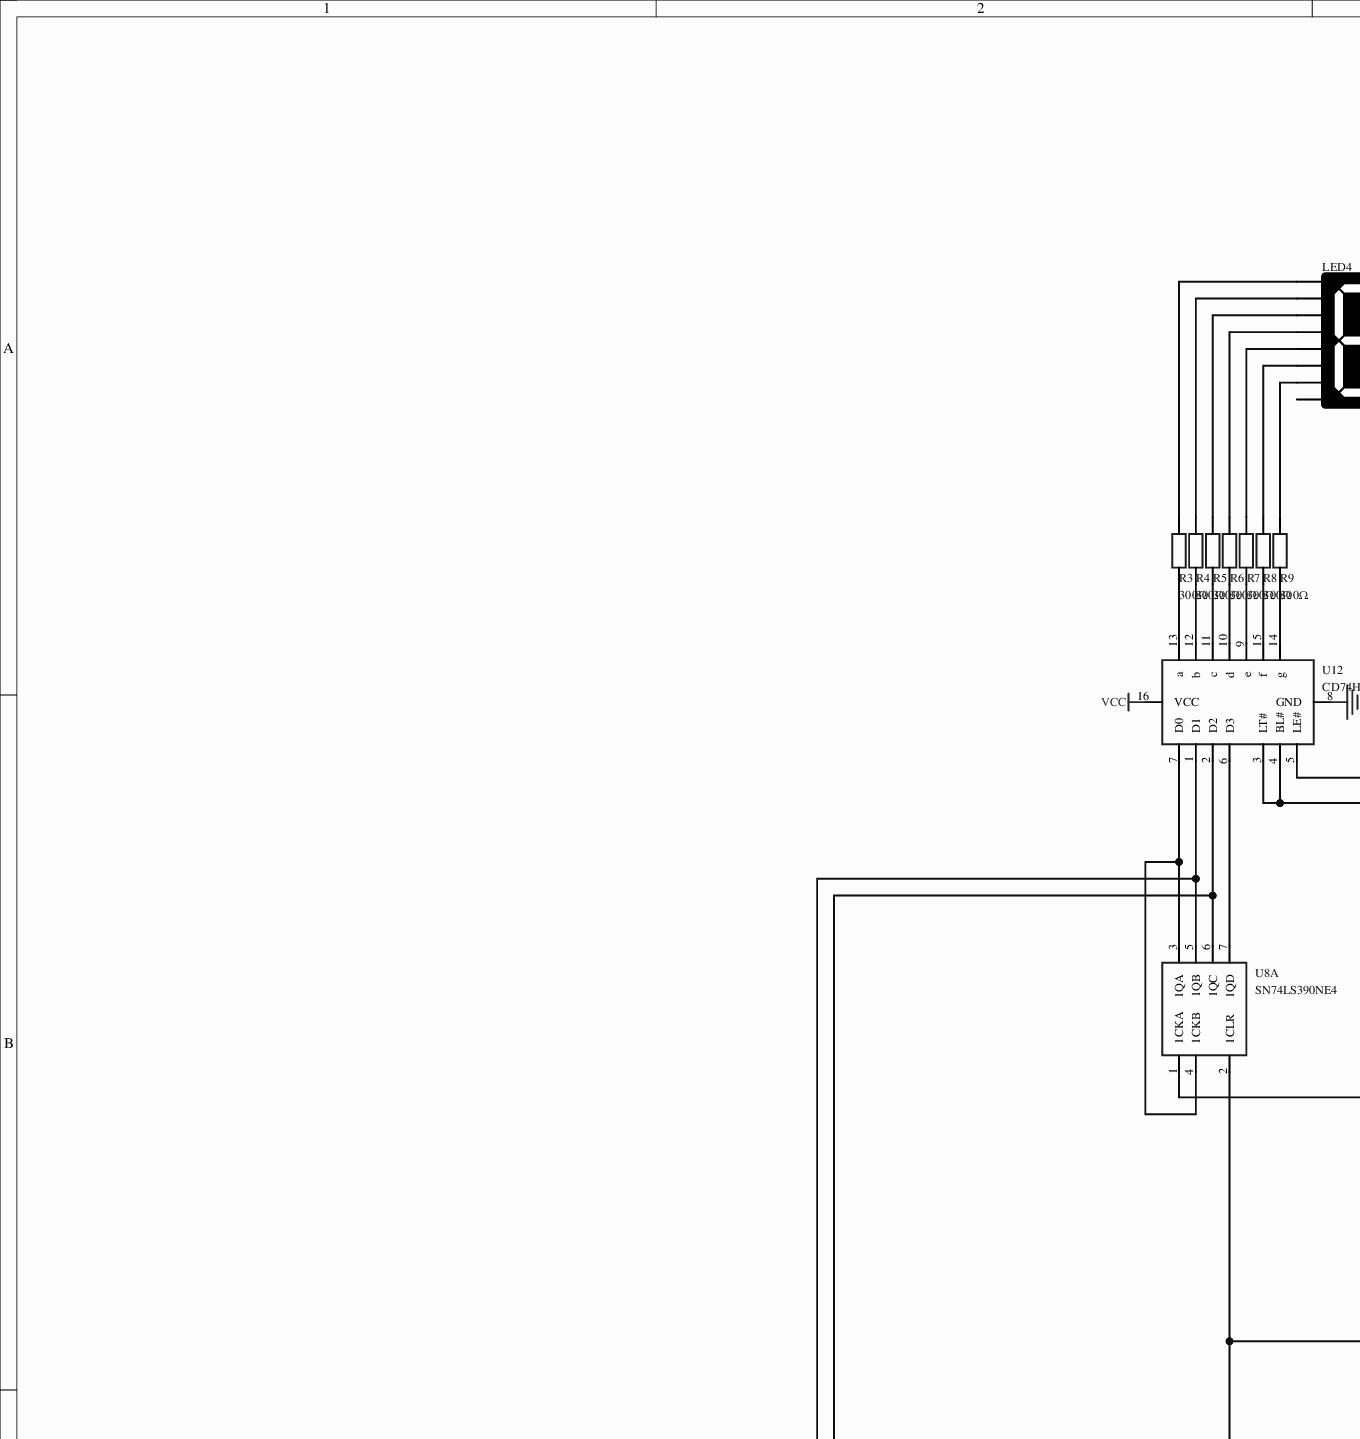
[diagram p0: MISC75414-3.schdoc, top left]
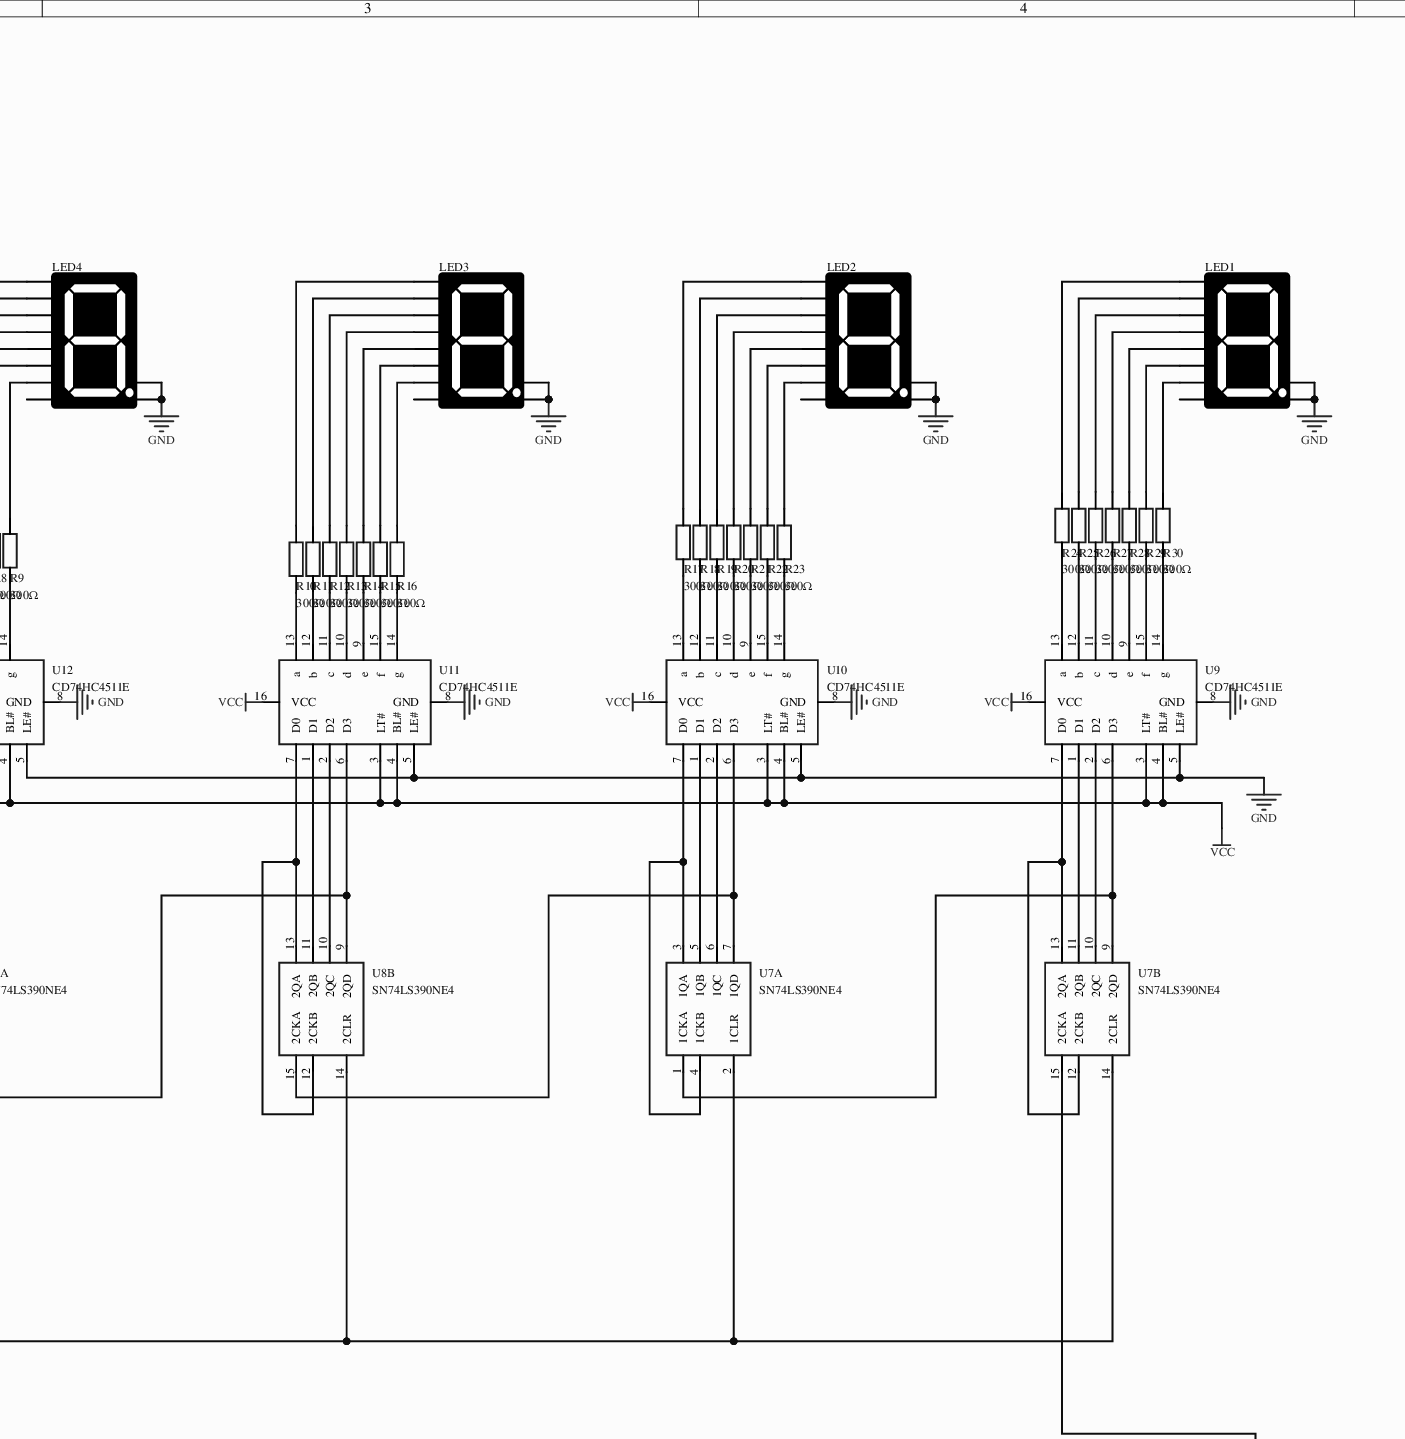
[diagram p1: MISC75414-3.schdoc, top middle]
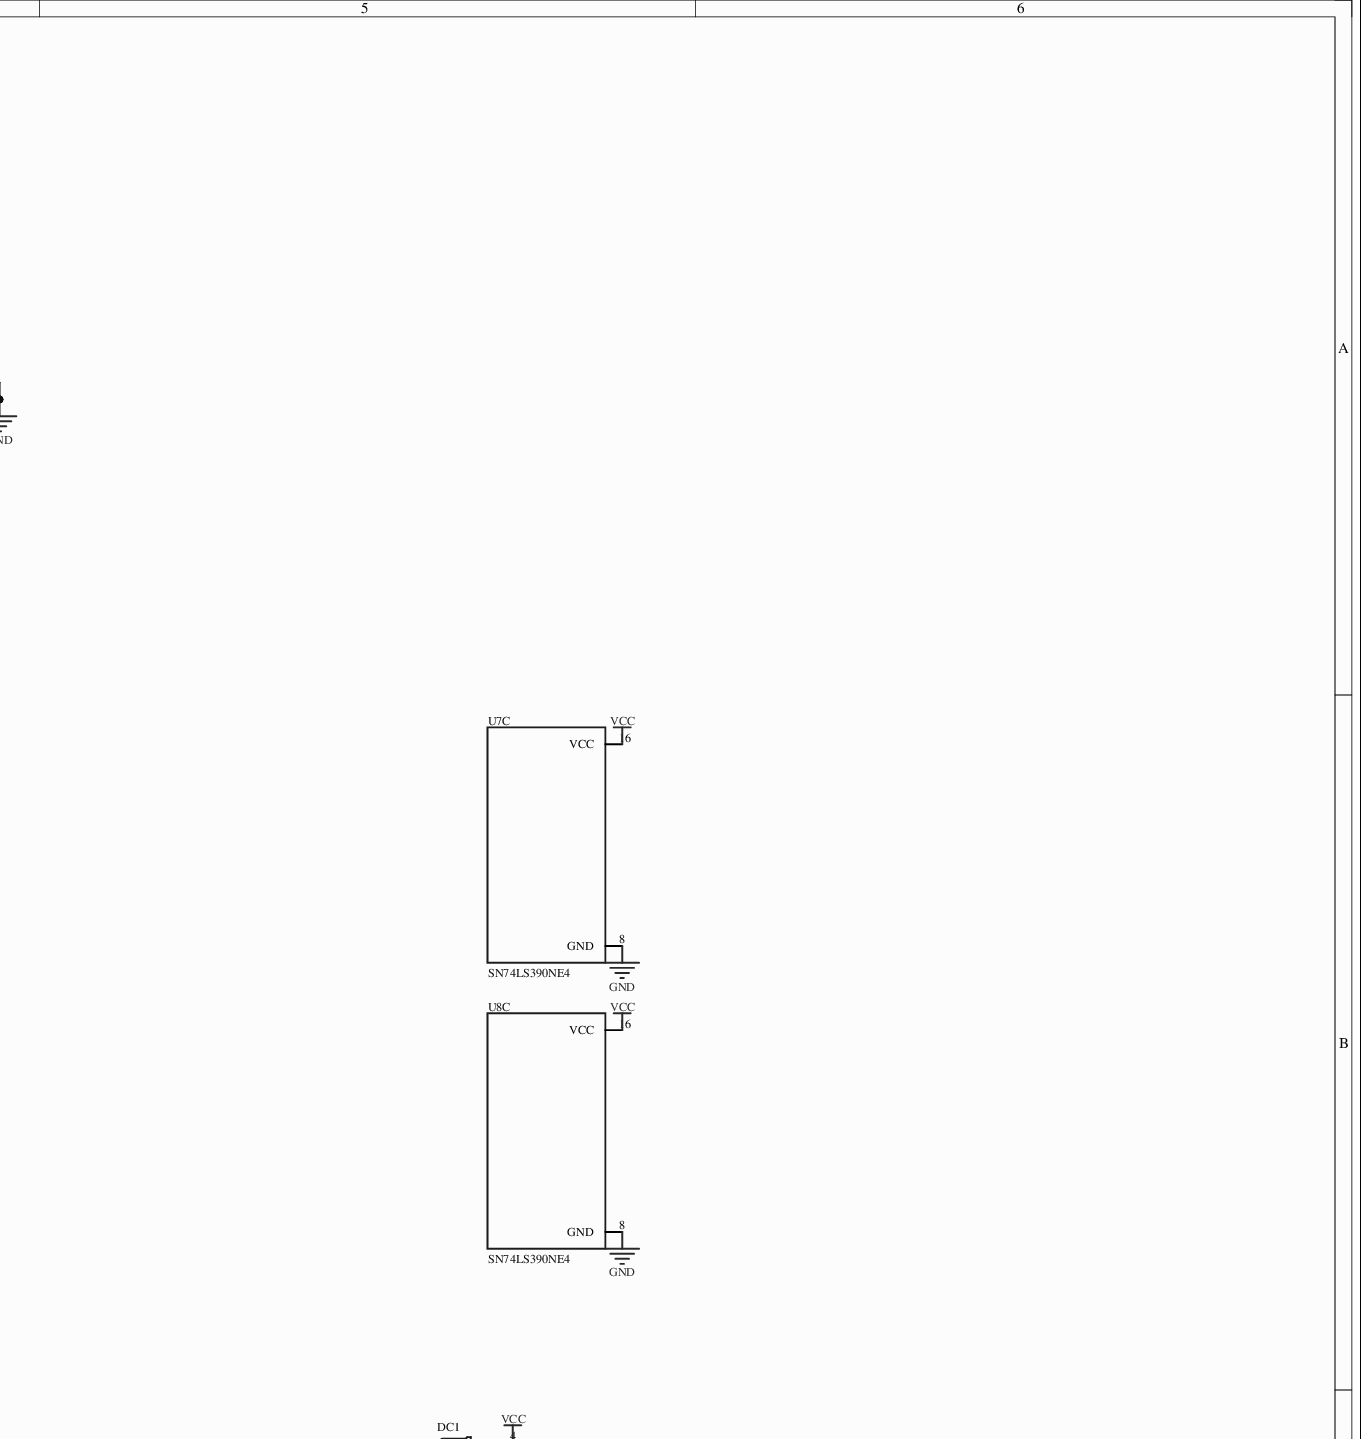
[diagram p2: MISC75414-3.schdoc, top right]
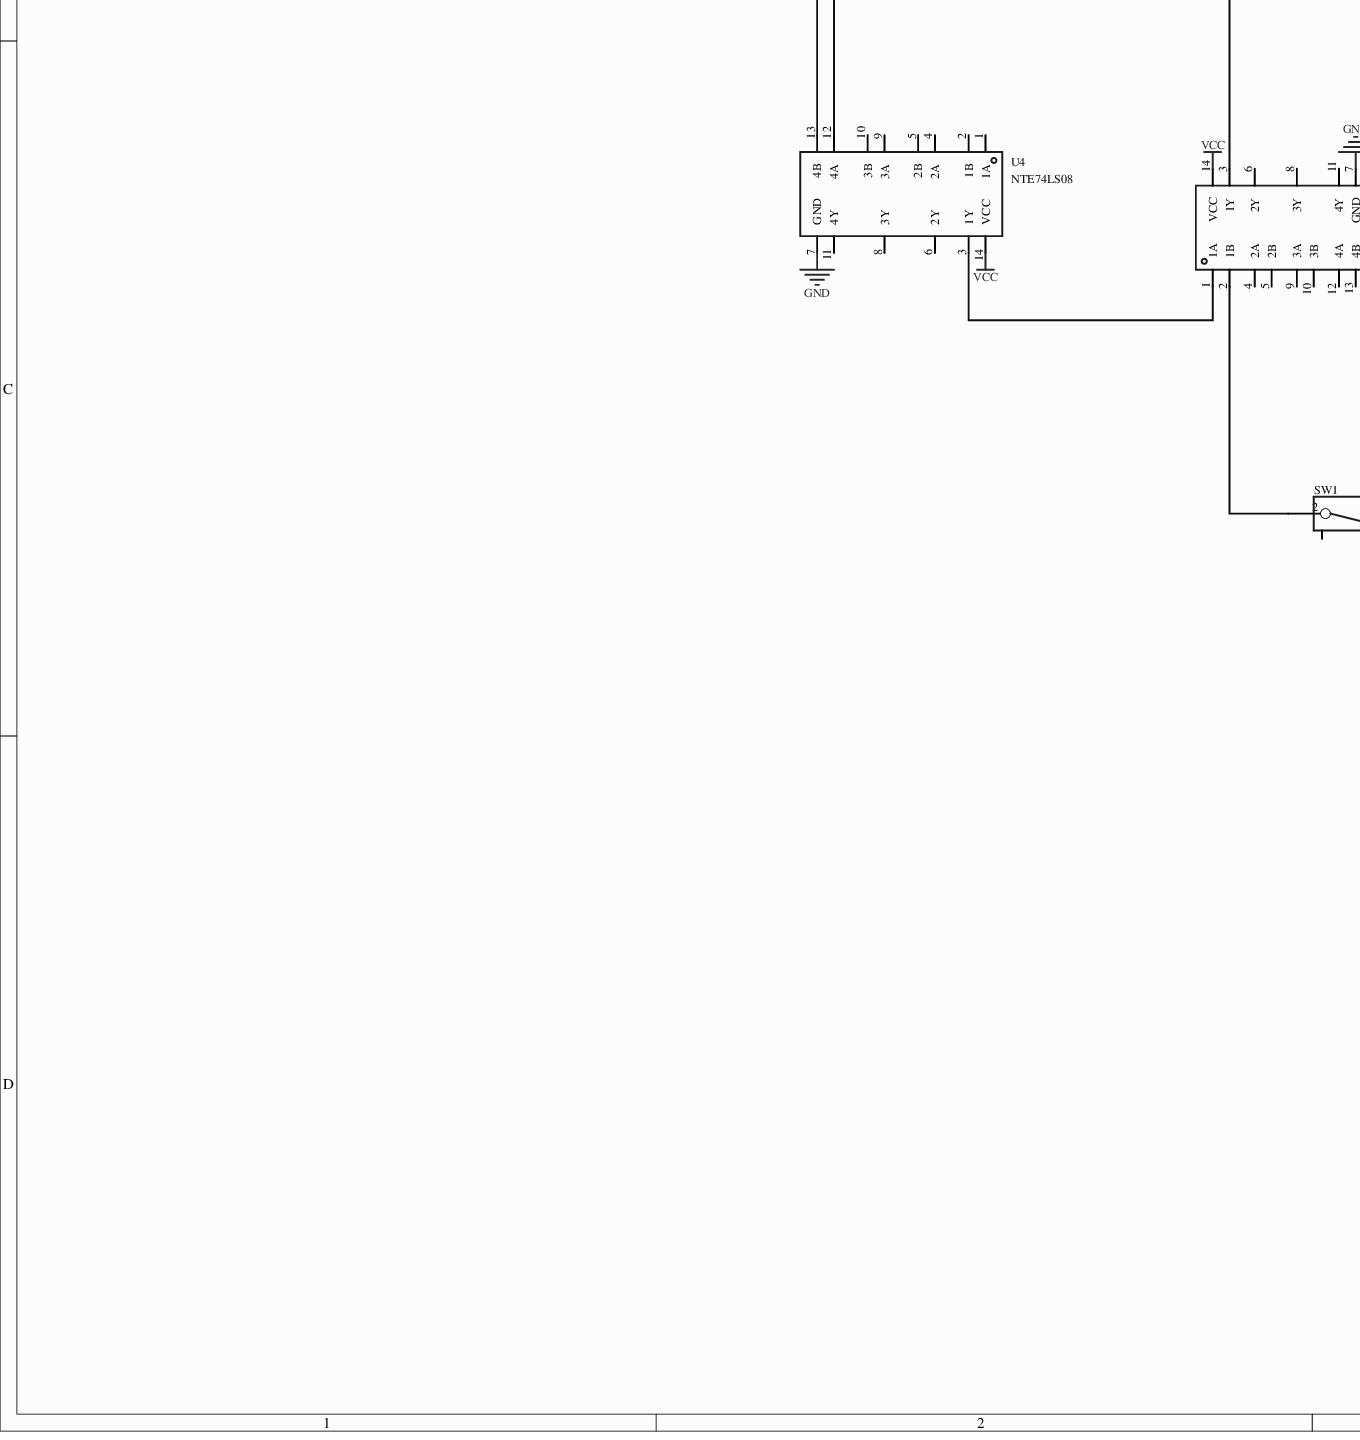
[diagram p3: MISC75414-3.schdoc, bottom left]
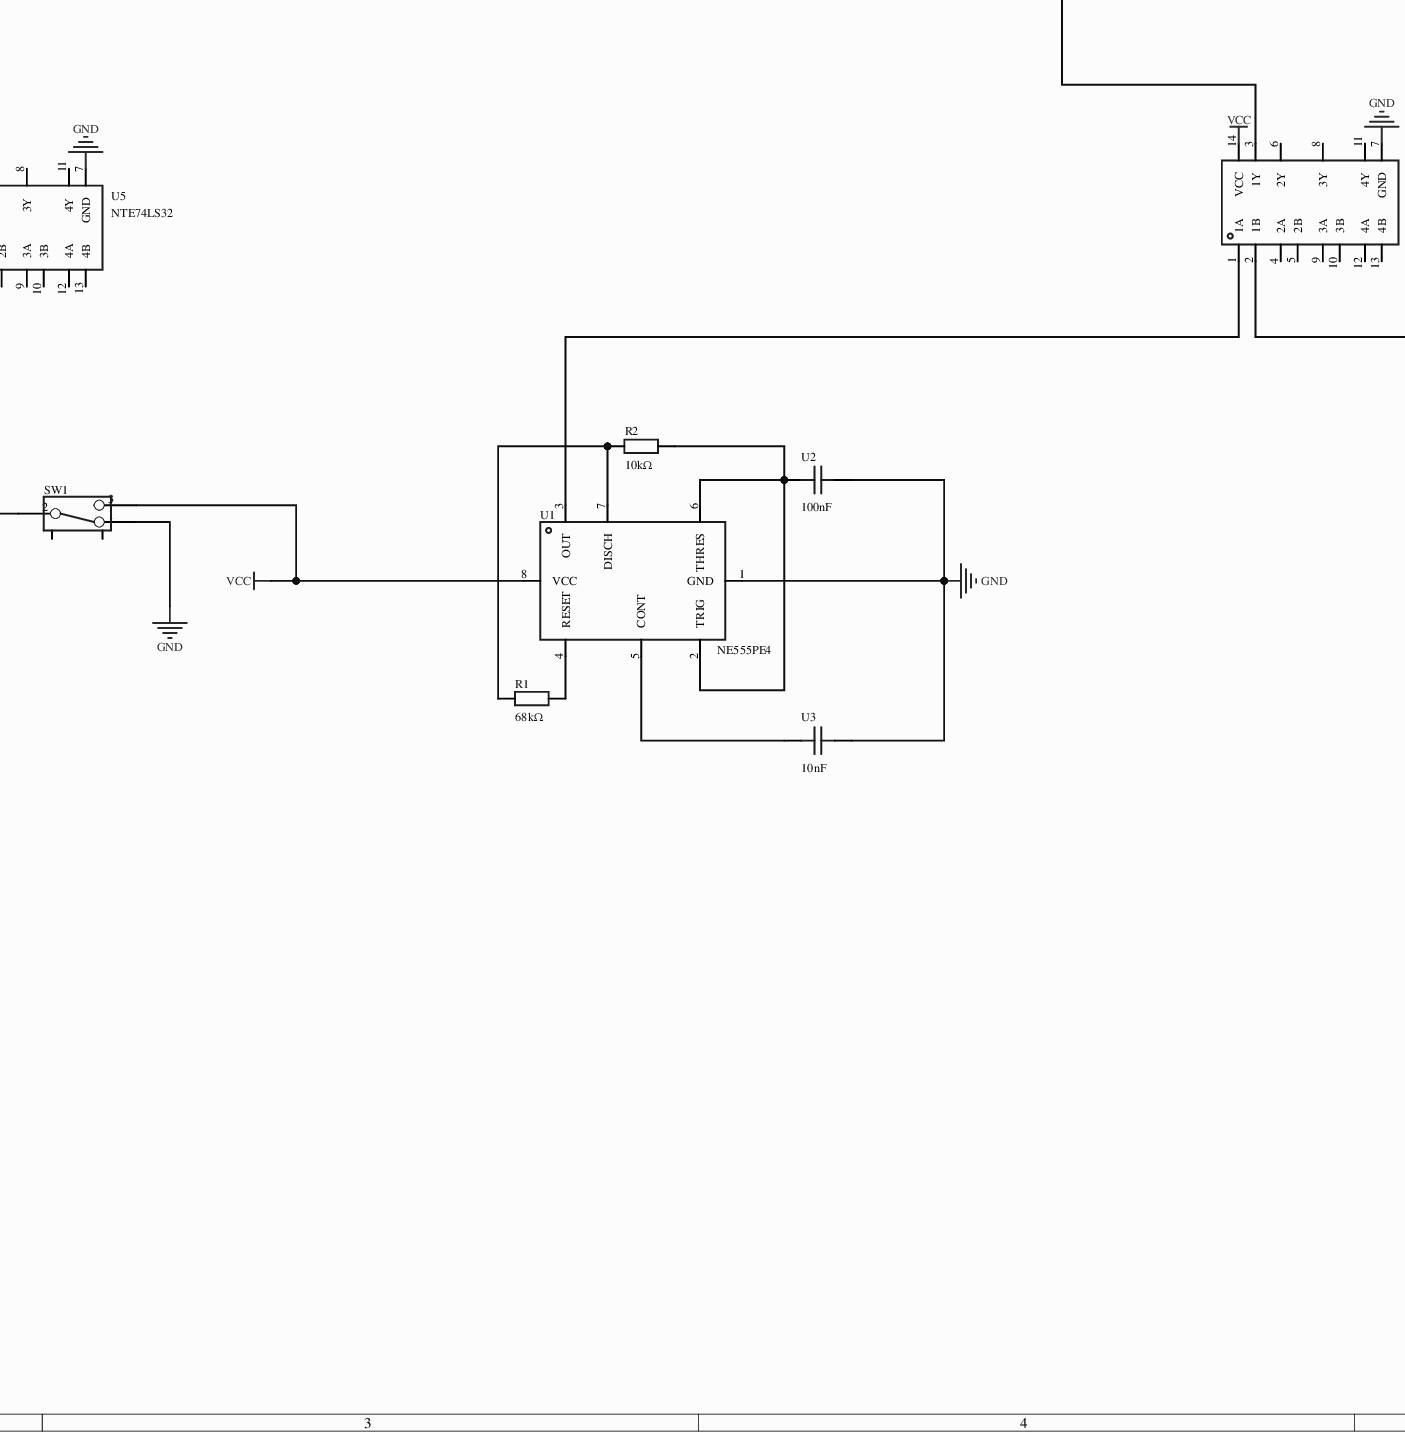
[diagram p4: MISC75414-3.schdoc, bottom middle]
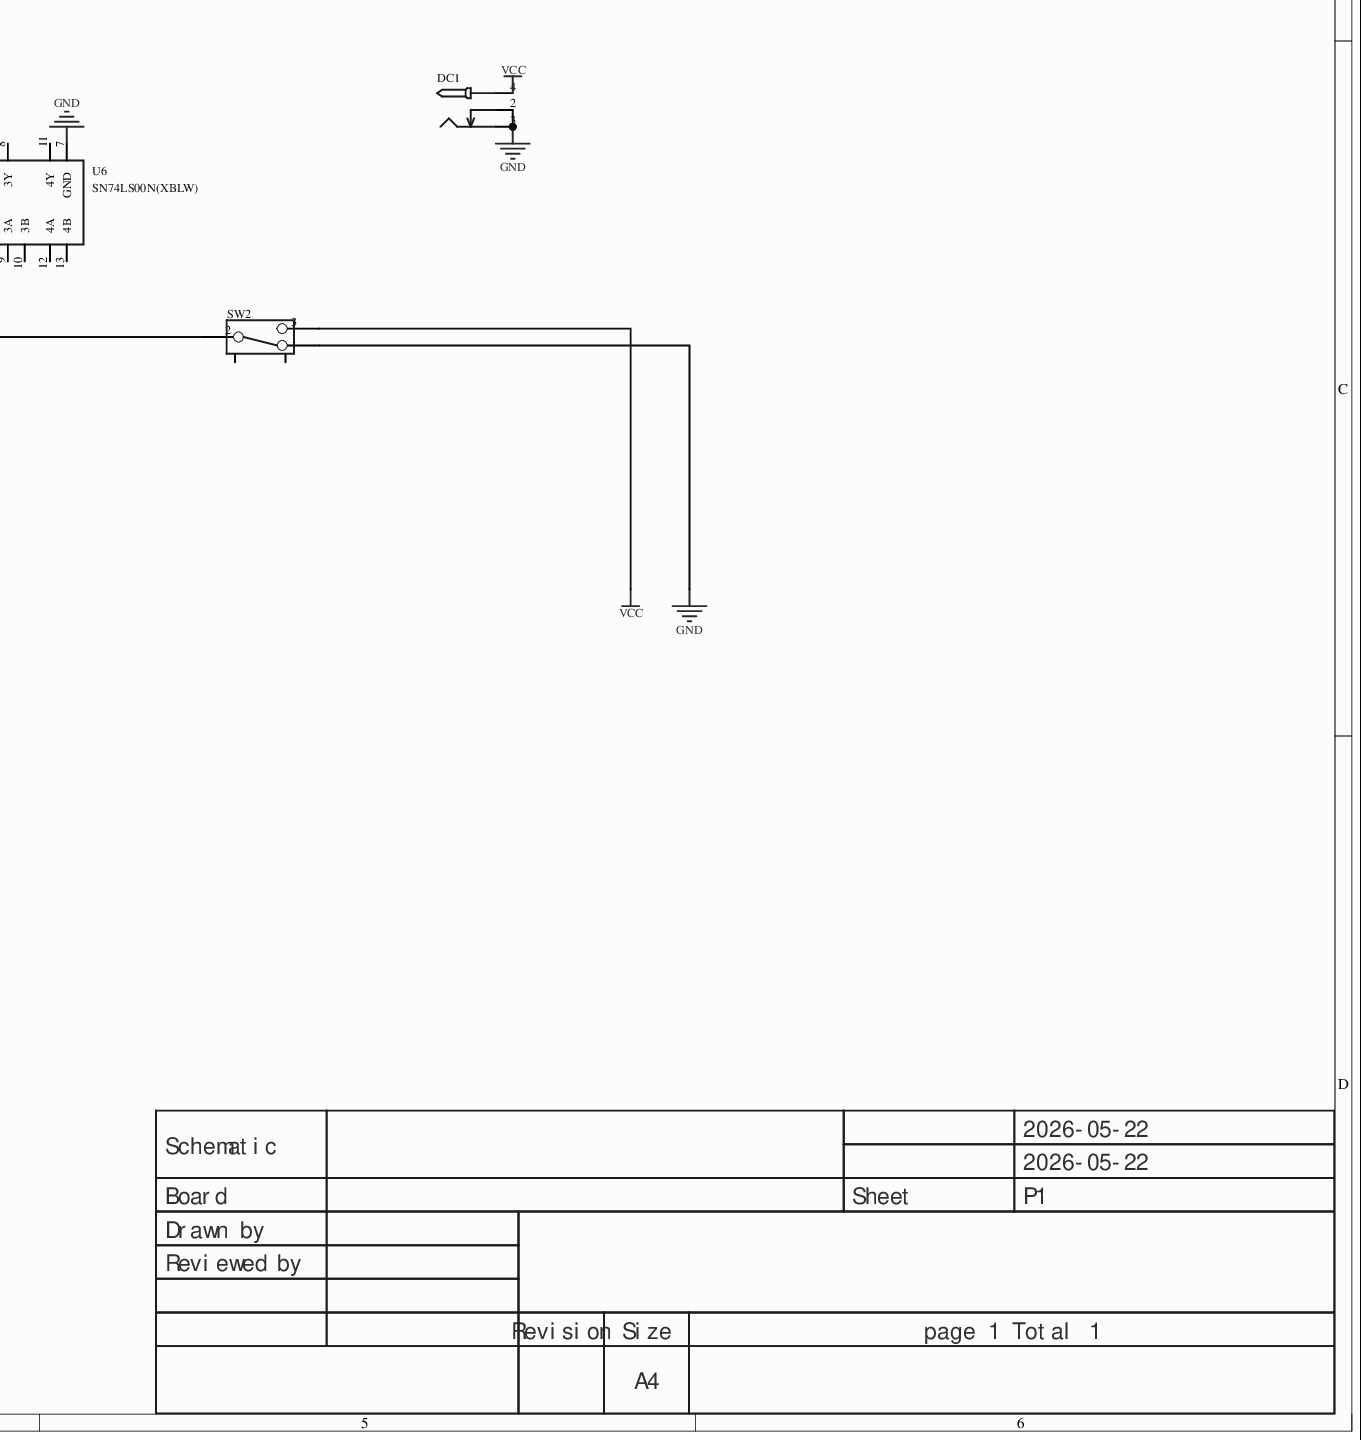
[diagram p5: MISC75414-3.schdoc, bottom right]
# Altium project MISC75414-2.PrjPcb
1 sheet, 49 parts. Net scope: global (net labels, ports and power ports of the same name join across sheets).
Board file: MISC75414.pcbdoc

## Sheet MISC75414-3.schdoc
size 594 x 419 mm; Version: V1.0; @Project Name: MISC75414; @Update Date: 2026-05-22; @Create Date: 2026-05-22; @Board Name: MISC75414; @Create Time: 21:43:26; @Page Count: 1; @Page No: 1; @Schematic Name: MISC75414; @Update Time: 21:43:26; Size: A4

### Parts
DC1  (no value)  [DC-2.0]
LED1  (no value)  [LED-SEG-TH_10P-L12.6-W19.0-P2.54-S15.24-BL]
LED2  (no value)  [LED-SEG-TH_10P-L12.6-W19.0-P2.54-S15.24-BL]
LED3  (no value)  [LED-SEG-TH_10P-L12.6-W19.0-P2.54-S15.24-BL]
LED4  (no value)  [LED-SEG-TH_10P-L12.6-W19.0-P2.54-S15.24-BL]
R1  68kΩ  [Res_1/8W]
R2  10kΩ  [Res_1/8W]
R3  300Ω  [Res_1/8W]
R4  300Ω  [Res_1/8W]
R5  300Ω  [Res_1/8W]
R6  300Ω  [Res_1/8W]
R7  300Ω  [Res_1/8W]
R8  300Ω  [Res_1/8W]
R9  300Ω  [Res_1/8W]
R10  300Ω  [Res_1/8W]
R11  300Ω  [Res_1/8W]
R12  300Ω  [Res_1/8W]
R13  300Ω  [Res_1/8W]
R14  300Ω  [Res_1/8W]
R15  300Ω  [Res_1/8W]
R16  300Ω  [Res_1/8W]
R17  300Ω  [Res_1/8W]
R18  300Ω  [Res_1/8W]
R19  300Ω  [Res_1/8W]
R20  300Ω  [Res_1/8W]
R21  300Ω  [Res_1/8W]
R22  300Ω  [Res_1/8W]
R23  300Ω  [Res_1/8W]
R24  300Ω  [Res_1/8W]
R25  300Ω  [Res_1/8W]
R26  300Ω  [Res_1/8W]
R27  300Ω  [Res_1/8W]
R28  300Ω  [Res_1/8W]
R29  300Ω  [Res_1/8W]
R30  300Ω  [Res_1/8W]
SW1  (no value)  [拨动开关_侧]
SW2  (no value)  [拨动开关_侧]
U1  NE555PE4  [PDIP-8_L9.6-W6.4-P2.54-LS7.9-BL-1]
U2  100nF  [CAP-TH_L5.0-W2.5-P5.00-D1.0]
U3  10nF  [CAP-TH_L5.0-W2.5-P5.00-D1.0]
U4  NTE74LS08  [DIP-14_L19.6-W6.4-P2.54-LS7.6-BL]
U5  NTE74LS32  [DIP-14_L19.6-W6.4-P2.54-LS7.6-BL]
U6  SN74LS00N(XBLW)  [PDIP-14_L19.3-W6.4-P2.54-LS7.6-BL]
U7  SN74LS390NE4  [PDIP-16_L19.3-W6.4-P2.54-LS7.94-BL]  (parts A,B,C of 3)
U8  SN74LS390NE4  [PDIP-16_L19.3-W6.4-P2.54-LS7.94-BL]  (parts A,B,C of 3)
U9  CD74HC4511E  [PDIP-16_L19.7-W6.6-P2.54-LS7.6-BL]
U10  CD74HC4511E  [PDIP-16_L19.7-W6.6-P2.54-LS7.6-BL]
U11  CD74HC4511E  [PDIP-16_L19.7-W6.6-P2.54-LS7.6-BL]
U12  CD74HC4511E  [PDIP-16_L19.7-W6.6-P2.54-LS7.6-BL]

### Nets
GND: DC1.2 DC1.3 LED1.3(G1) LED1.8(G2) LED2.3(G1) LED2.8(G2) LED3.3(G1) LED3.8(G2) LED4.3(G1) LED4.8(G2) SW1.1 SW2.1 U1.1(GND) U2.1 U3.1 U4.7(GND) U5.7(GND) U6.7(GND) U7.8(GND) U8.8(GND) U9.5(LE#) U9.8(GND) U10.5(LE#) U10.8(GND) U11.5(LE#) U11.8(GND) U12.5(LE#) U12.8(GND)
VCC: DC1.4 SW1.3 SW2.3 U1.8(VCC) U4.14(VCC) U5.14(VCC) U6.14(VCC) U7.16(VCC) U8.16(VCC) U9.3(LT#) U9.4(BL#) U9.16(VCC) U10.3(LT#) U10.4(BL#) U10.16(VCC) U11.3(LT#) U11.4(BL#) U11.16(VCC) U12.3(LT#) U12.4(BL#) U12.16(VCC)
NetLED1_1: LED1.1(E) R28.2
NetLED1_2: LED1.2(D) R27.2
NetLED1_4: LED1.4(C) R26.2
NetLED1_6: LED1.6(B) R25.2
NetLED1_7: LED1.7(A) R24.2
NetLED1_9: LED1.9(F) R29.2
NetLED1_10: LED1.10(G) R30.2
NetLED2_1: LED2.1(E) R21.2
NetLED2_2: LED2.2(D) R20.2
NetLED2_4: LED2.4(C) R19.2
NetLED2_6: LED2.6(B) R18.2
NetLED2_7: LED2.7(A) R17.2
NetLED2_9: LED2.9(F) R22.2
NetLED2_10: LED2.10(G) R23.2
NetLED3_1: LED3.1(E) R14.2
NetLED3_2: LED3.2(D) R13.2
NetLED3_4: LED3.4(C) R12.2
NetLED3_6: LED3.6(B) R11.2
NetLED3_7: LED3.7(A) R10.2
NetLED3_9: LED3.9(F) R15.2
NetLED3_10: LED3.10(G) R16.2
NetLED4_1: LED4.1(E) R7.2
NetLED4_2: LED4.2(D) R6.2
NetLED4_4: LED4.4(C) R5.2
NetLED4_6: LED4.6(B) R4.2
NetLED4_7: LED4.7(A) R3.2
NetLED4_9: LED4.9(F) R8.2
NetLED4_10: LED4.10(G) R9.2
NetR1_1: R1.1 R2.1 U1.7(DISCH)
NetR1_2: R1.2 U1.4(RESET)
NetR2_2: R2.2 U1.2(TRIG) U1.6(THRES) U2.2
NetR3_1: R3.1 U12.13(a)
NetR4_1: R4.1 U12.12(b)
NetR5_1: R5.1 U12.11(c)
NetR6_1: R6.1 U12.10(d)
NetR7_1: R7.1 U12.9(e)
NetR8_1: R8.1 U12.15(f)
NetR9_1: R9.1 U12.14(g)
NetR10_1: R10.1 U11.13(a)
NetR11_1: R11.1 U11.12(b)
NetR12_1: R12.1 U11.11(c)
NetR13_1: R13.1 U11.10(d)
NetR14_1: R14.1 U11.9(e)
NetR15_1: R15.1 U11.15(f)
NetR16_1: R16.1 U11.14(g)
NetR17_1: R17.1 U10.13(a)
NetR18_1: R18.1 U10.12(b)
NetR19_1: R19.1 U10.11(c)
NetR20_1: R20.1 U10.10(d)
NetR21_1: R21.1 U10.9(e)
NetR22_1: R22.1 U10.15(f)
NetR23_1: R23.1 U10.14(g)
NetR24_1: R24.1 U9.13(a)
NetR25_1: R25.1 U9.12(b)
NetR26_1: R26.1 U9.11(c)
NetR27_1: R27.1 U9.10(d)
NetR28_1: R28.1 U9.9(e)
NetR29_1: R29.1 U9.15(f)
NetR30_1: R30.1 U9.14(g)
NetSW1_2: SW1.2 U5.2(1B)
NetSW2_2: SW2.2 U6.2(1B)
NetU1_3: U1.3(OUT) U6.1(1A)
NetU1_5: U1.5(CONT) U3.2
NetU4_3: U4.3(1Y) U5.1(1A)
NetU4_12: U4.12(4A) U8.6(1QC) U12.2(D2)
NetU4_13: U4.13(4B) U8.5(1QB) U12.1(D1)
NetU5_3: U5.3(1Y) U7.2(1CLR) U7.14(2CLR) U8.2(1CLR) U8.14(2CLR)
NetU6_3: U6.3(1Y) U7.15(2CKA)
NetU7_1: U7.1(1CKA) U7.9(2QD) U9.6(D3)
NetU7_3: U7.3(1QA) U7.4(1CKB) U10.7(D0)
NetU7_5: U7.5(1QB) U10.1(D1)
NetU7_6: U7.6(1QC) U10.2(D2)
NetU7_7: U7.7(1QD) U8.15(2CKA) U10.6(D3)
NetU7_10: U7.10(2QC) U9.2(D2)
NetU7_11: U7.11(2QB) U9.1(D1)
NetU7_12: U7.12(2CKB) U7.13(2QA) U9.7(D0)
NetU8_1: U8.1(1CKA) U8.9(2QD) U11.6(D3)
NetU8_3: U8.3(1QA) U8.4(1CKB) U12.7(D0)
NetU8_7: U8.7(1QD) U12.6(D3)
NetU8_10: U8.10(2QC) U11.2(D2)
NetU8_11: U8.11(2QB) U11.1(D1)
NetU8_12: U8.12(2CKB) U8.13(2QA) U11.7(D0)

Not connected (* = marked no-connect by the designer): LED1 5(DP); LED2 5(DP); LED3 5(DP); LED4 5(DP); SW1 4 5; SW2 4 5; U4 1(1A) 2(1B) 4(2A) 5(2B) 6(2Y) 8(3Y) 9(3A) 10(3B) 11(4Y); U5 4(2A) 5(2B) 6(2Y) 8(3Y) 9(3A) 10(3B) 11(4Y) 12(4A) 13(4B); U6 4(2A) 5(2B) 6(2Y) 8(3Y) 9(3A) 10(3B) 11(4Y) 12(4A) 13(4B)

### Notes on the sheet
- 2026-05-22
- Schematic
- Board
- Sheet
- P1
- Drawn by
- Reviewed by
- Revision
- Size
- A4
- page 1 Total 1

### Library data of the parts
DC1 = DC-005_2.0: Symbol: DC power connector; ConvertToPcb: yes; ModelId: f5f20b8a2308479b936ba3c2698865bb0819f05c4eef4c71ace90d822a990e87; ModelName: DC-IN-TH_DC-5520-1; ModelTransform: 372.05,551.18,582.68,90,0,0,137.8,0,-149.61; Device: DC-005_2.0; AddInBom: yes; Supplier Footprint: 插件; FootprintName: DC-2.0
LED1-LED4 = LED_SEG_TH_0.56x1: Symbol: LED_SEG_TH_0.56*1; ConvertToPcb: yes; ModelId: 16c3aae6d39e4ecc9e744d6eeac8d57b0819f05c4eef4c71ace90d822a990e87; ModelName: LED-SEG-TH_0.56_1p; ModelTransform: 496.062,748.03,0,0,0,0,0,0,-137.795; Device: LED_SEG_TH_0.56x1; AddInBom: yes; Supplier Footprint: 插件; FootprintName: LED-SEG-TH_10P-L12.6-W19.0-P2.54-S15.24-BL
R1 R2 = Res_AXIAL-1/8W: Symbol: Resistor; ConvertToPcb: yes; ModelId: b2b5ae7ae4c642178fe0039925c86a3f0819f05c4eef4c71ace90d822a990e87; ModelName: RES-TH_BD1.8-L3.2-P7.20-D0.4; ModelTransform: 282.86,66.88,253.09,0,0,0,0,0,-191; Device: Res_AXIAL-1/8W; AddInBom: yes; Supplier Footprint: 轴向引线; FootprintName: Res_1/8W
  R1: Value: 68kΩ
  R2: Value: 10kΩ
R3-R30 = Res_AXIAL-1/8W: Symbol: Resistor; 3D Model: b2b5ae7ae4c642178fe0039925c86a3f0819f05c4eef4c71ace90d822a990e87; 3D Model Transform: 282.86,66.88,253.09,0,0,0,0,0,-191; ConvertToPcb: yes; ModelName: RES-TH_BD1.8-L3.2-P7.20-D0.4; Device: Res_AXIAL-1/8W; Supplier Footprint: 轴向引线; Value: 300Ω; AddInBom: yes; FootprintName: Res_1/8W
SW1 SW2 = 拨动开关_侧: Symbol: Toggle switch; Device: Toggle switch, side; ConvertToPcb: yes; ModelId: 10ea2cc5ba004a75b38812aadef1031f0819f05c4eef4c71ace90d822a990e87; ModelName: SW-TH_SK-12D07-VG3; ModelTransform: 337.98,287.46,295.24,0,0,0,0,-57,-110; AddInBom: yes; Supplier Footprint: 插件; FootprintName: Toggle switch, side
U1 = NE555PE4: NE555 single timer; Manufacturer: TI(德州仪器); AddInBom: yes; ModelId: 1b8eaf096e7944deafe216467068c10e0819f05c4eef4c71ace90d822a990e87; ModelTransform: 377.952,318.897,0,0,0,0,0,0,-118.11; Symbol: NE555PE4; Device: NE555PE4; LCSC Part Name: NE555PE4; SupplierPart: C2859604; ManufacturerPart: NE555PE4; Supplier Footprint: PDIP-8; JLCPCB Part Class: Extended Part; Datasheet: https://www.ti.com/cn/lit/gpn/sa555; Supplier: LCSC; ConvertToPcb: yes; FootprintName: PDIP-8_L9.6-W6.4-P2.54-LS7.9-BL-1; ModelName: PDIP-8_L9.6-W6.4-P2.54-LS7.9-BL-1
U2 U3 = 100nF: Symbol: 100NF_C9900015256; AddInBom: yes; ModelId: 08e3d7481fc7486bb1b263873f51e1e10819f05c4eef4c71ace90d822a990e87; ModelName: CAP-TH_BD5.0-W2.5-P5.08; ModelTransform: 224.652,98.425,0,0,0,0,-0.005,0,-137.795; Device: 100nF; LCSC Part Name: 100nF; SupplierPart: C9900015256; Supplier Footprint: CAP-TH_L5.0-W2.5-P5.00-D1.0; JLCPCB Part Class: Extended Part; Supplier: LCSC; ConvertToPcb: yes; FootprintName: CAP-TH_L5.0-W2.5-P5.00-D1.0
  U2: ManufacturerPart: 100nF
  U3: Manufacturer Part: 10nF
U4 = NTE74LS08: Logic type: AND gate; channels: 4; operating voltage: 4.75V~5.25V; quiescent current (Iq): 8.8mA; propagation delay (tpd): 20ns@5V,15pF;; Manufacturer: NTE ELECTRONICS, INC.; AddInBom: yes; ModelId: 0519cdc58ae14e7f86534804b9ac5d8e0819f05c4eef4c71ace90d822a990e87; ModelTransform: 769.6835,309.842,0,0,0,0,0,0,-137.795; Number of Channels: 4; Current - Output Low(IOL): 8mA; Current - Output High(IOH): 400uA; Input Logic Level - High: 2V; Input Logic Level - Low: 800mV; Symbol: NTE74LS08; Device: NTE74LS08; LCSC Part Name: NTE74LS08; SupplierPart: C6944031; ManufacturerPart: NTE74LS08; Supplier Footprint: PDIP-14; JLCPCB Part Class: Extended Part; Datasheet: https://atta.szlcsc.com/upload/public/pdf/source/231023/nte74LS08.pdf-33fda59c8c58886a1fb84369fc2a9978.pdf; Supplier: LCSC; ConvertToPcb: yes; FootprintName: DIP-14_L19.6-W6.4-P2.54-LS7.6-BL; ModelName: DIP-14_L19.6-W6.4-P2.54-LS7.6-BL; Logic Type: AND gate; Voltage - Supply: 4.75V~5.25V; Quiescent Current: 8.8mA; Propagation Delay: 20ns@5V,15pF; Operating Temperature: 0℃~+70℃
U5 = NTE74LS32: Logic type: OR gate; channels: 4; operating voltage: 4.75V~5.25V; propagation delay (tpd): 22ns@5V,50pF;; Manufacturer: NTE ELECTRONICS, INC.; AddInBom: yes; ModelId: 0519cdc58ae14e7f86534804b9ac5d8e0819f05c4eef4c71ace90d822a990e87; ModelTransform: 769.6835,309.842,0,0,0,0,0,0,-137.795; Logic Type: OR gate; Number of Channels: 4; Current - Output Low(IOL): 8mA; Current - Output High(IOH): 400uA; Input Logic Level - High: 2V; Input Logic Level - Low: 800mV; Symbol: NTE74LS32; Device: NTE74LS32; LCSC Part Name: NTE74LS32; SupplierPart: C6134262; ManufacturerPart: NTE74LS32; Supplier Footprint: DIP-14; JLCPCB Part Class: Extended Part; Datasheet: https://atta.szlcsc.com/upload/public/pdf/source/231023/nte74LS32.pdf-f7bcd142ccb75874952b6adc8cab0905.pdf; Supplier: LCSC; ConvertToPcb: yes; FootprintName: DIP-14_L19.6-W6.4-P2.54-LS7.6-BL; ModelName: DIP-14_L19.6-W6.4-P2.54-LS7.6-BL; Voltage - Supply: 4.75V~5.25V; Series: 74LS series; Propagation Delay: 22ns@5V,50pF; Operating Temperature: 0℃~+70℃
U6 = SN74LS00N(XBLW): SN74LS00 is a quad 2-input NAND gate; inputs include clamp diodes, allowing current-limiting resistors to interface inputs to voltages above Vcc.; Manufacturer: XBLW(芯伯乐); AddInBom: yes; ModelId: ca4ed987146b49a5a2d3ca847d6466c40819f05c4eef4c71ace90d822a990e87; ModelTransform: 755.904,309.842,0,0,0,0,0,0,-125.984; Symbol: SN74LS00N(XBLW); Device: SN74LS00N(XBLW); LCSC Part Name: 四路二输入与非门; SupplierPart: C42395504; ManufacturerPart: SN74LS00N(XBLW); Supplier Footprint: DIP-14; JLCPCB Part Class: Extended Part; Datasheet: https://item.szlcsc.com/datasheet/SN74LS00N(XBLW)/44341338.html; Supplier: LCSC; ConvertToPcb: yes; FootprintName: PDIP-14_L19.3-W6.4-P2.54-LS7.6-BL; ModelName: PDIP-14_L19.3-W6.4-P2.54-LS7.6-BL
U7 = SN74LS390NE4: SN74LS390 dual 4-bit decade counter; Manufacturer: TI(德州仪器); Add into BOM: yes; 3D Model: 96ff5d01b3074dd183bcbc4cd00a63de0819f05c4eef4c71ace90d822a990e87; 3D Model Transform: 759.841,322.44,0,0,0,0,0,0,-137.795; Symbol: SN74LS390NE4; Device: SN74LS390NE4; Convert to PCB: yes; LCSC Part Name: 双4位十进制和二进制计数器; Supplier Part: C20345771; Manufacturer Part: SN74LS390NE4; Supplier Footprint: PDIP-16; JLCPCB Part Class: Extended Part; Datasheet: https://item.szlcsc.com/datasheet/SN74LS390NE4/21671298.html; Supplier: LCSC; FootprintName: PDIP-16_L19.3-W6.4-P2.54-LS7.94-BL; ModelName: PDIP-16_L19.3-W6.4-P2.54-LS7.94-BL
U8 = SN74LS390NE4: SN74LS390 dual 4-bit decade counter; Manufacturer: TI(德州仪器); Relevance: []; Add into BOM: yes; 3D Model: 96ff5d01b3074dd183bcbc4cd00a63de0819f05c4eef4c71ace90d822a990e87; 3D Model Transform: 759.841,322.44,0,0,0,0,0,0,-137.795; Symbol: SN74LS390NE4; Device: SN74LS390NE4; Convert to PCB: yes; LCSC Part Name: 双4位十进制和二进制计数器; Supplier Part: C20345771; Manufacturer Part: SN74LS390NE4; Supplier Footprint: PDIP-16; JLCPCB Part Class: Extended Part; Datasheet: https://item.szlcsc.com/datasheet/SN74LS390NE4/21671298.html; Supplier: LCSC; FootprintName: PDIP-16_L19.3-W6.4-P2.54-LS7.94-BL; ModelName: PDIP-16_L19.3-W6.4-P2.54-LS7.94-BL
U9-U12 = CD74HC4511E: CD74HC4511 high-speed CMOS logic BCD to 7-segment latch/decoder/driver; Manufacturer: TI(德州仪器); AddInBom: yes; ModelId: 60304d8eb9b246fdb135cb3d16f241a80819f05c4eef4c71ace90d822a990e87; ModelName: PDIP-16_L19.7-W6.6-H5.1-P2.54-LS7.6-BL; ModelTransform: 787.4,311.8104,0,0,0,0,0,0,-118.11; Symbol: CD74HC4511E; Device: CD74HC4511E; LCSC Part Name: CD74HC4511E; SupplierPart: C1524046; ManufacturerPart: CD74HC4511E; Supplier Footprint: PDIP-16; JLCPCB Part Class: Extended Part; Datasheet: https://www.ti.com/cn/lit/gpn/cd74hc4511; Supplier: LCSC; ConvertToPcb: yes; FootprintName: PDIP-16_L19.7-W6.6-P2.54-LS7.6-BL